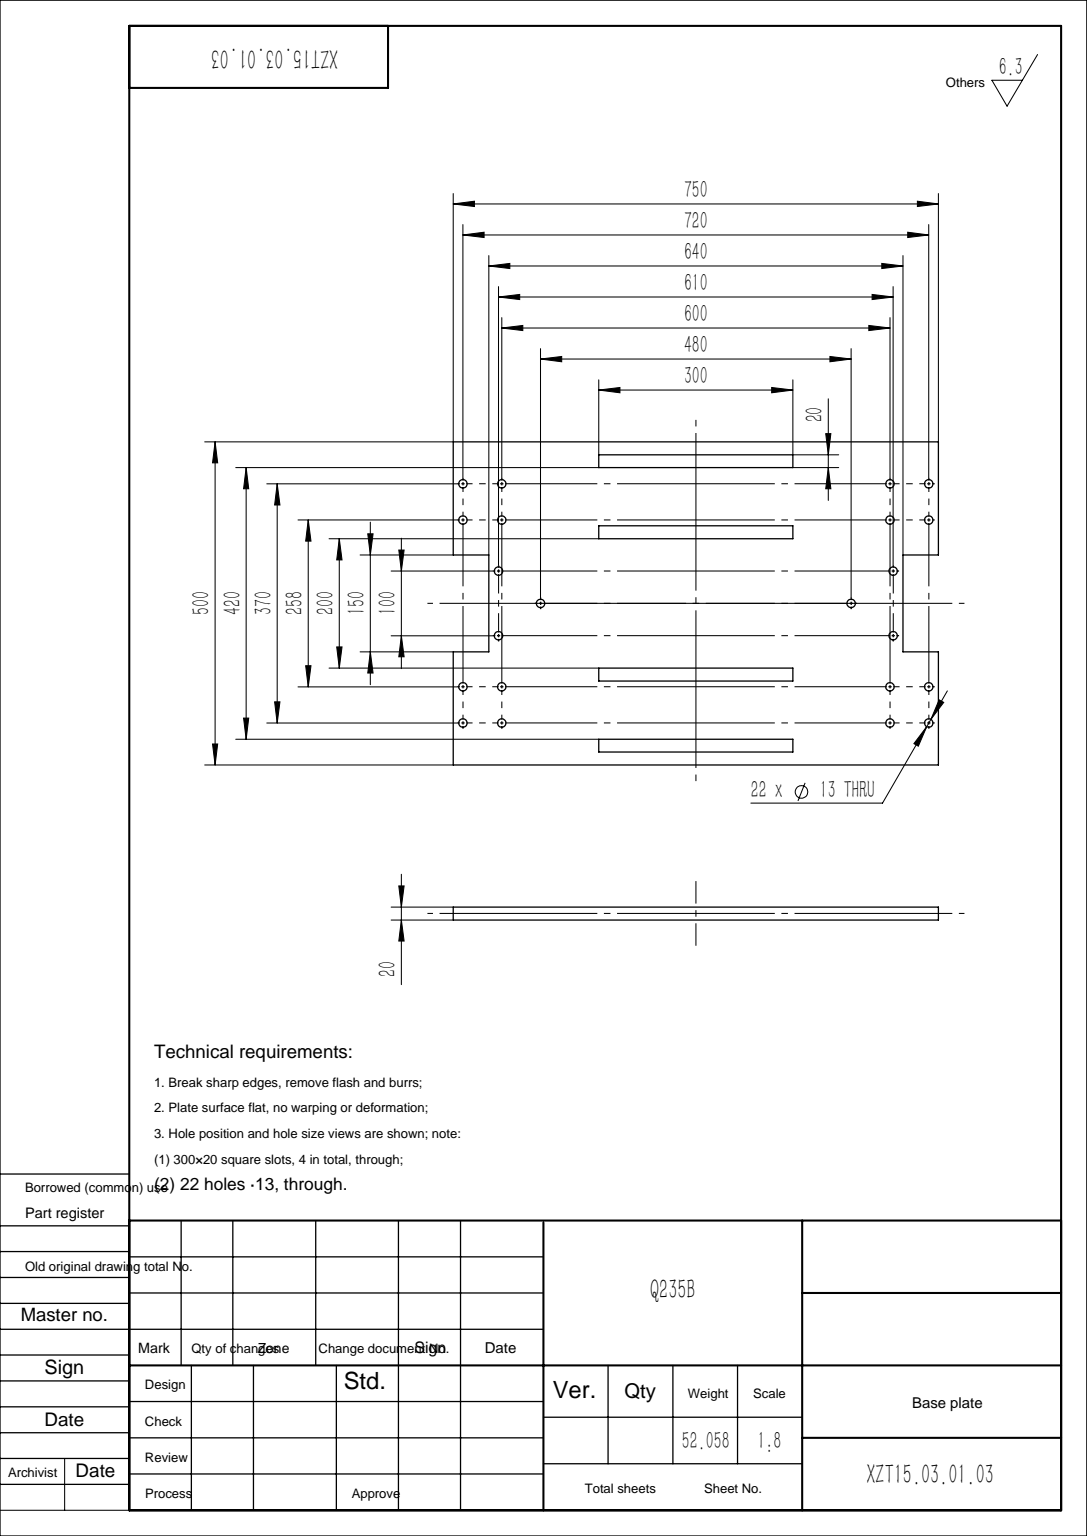
SolidWorks part; units mm, degrees
material "Q235B"
ref_plane "Front Plane" through (0, 0, 0) normal (0, 0, 1) x (1, 0, 0)
ref_plane "Top Plane" through (0, 0, 0) normal (0, 1, 0) x (1, 0, 0)
ref_plane "Right Plane" through (0, 0, 0) normal (1, 0, 0) x (0, 0, -1)
sketch "Sketch1" plane through (0, 0, 0) normal (0, 1, 0) x (1, 0, 0)
  line L0 (0, 0) -> (0, 250) construction
  line L1 (375, -250) -> (-375, -250)
  line L2 (375, -250) -> (375, 250)
  line L3 (375, 250) -> (-375, 250)
  line L4 (-375, -250) -> (-375, 250)
  line L5 (375, -250) -> (-375, 250) construction
  line L6 (375, 250) -> (-375, -250) construction
  line L7 (-320, -75) -> (-430, -75)
  line L8 (-320, -75) -> (-320, 75)
  line L9 (-320, 75) -> (-430, 75)
  line L10 (-430, -75) -> (-430, 75)
  line L11 (-320, -75) -> (-430, 75) construction
  line L12 (-320, 75) -> (-430, -75) construction
  line L13 (0, 0) -> (375, 0) construction
  line L14 (150, -120) -> (-150, -100) construction
  line L15 (150, 210) -> (-150, 210)
  line L16 (150, 210) -> (150, 230)
  line L17 (150, 230) -> (-150, 230)
  line L18 (-150, 210) -> (-150, 230)
  line L19 (150, 210) -> (-150, 230) construction
  line L20 (150, 230) -> (-150, 210) construction
  line L21 (150, 100) -> (-150, 100)
  line L22 (150, 100) -> (150, 120)
  line L23 (150, 120) -> (-150, 120)
  line L24 (-150, 100) -> (-150, 120)
  line L25 (150, 100) -> (-150, 120) construction
  line L26 (150, 120) -> (-150, 100) construction
  line L27 (150, -100) -> (-150, -120) construction
  line L28 (150, -230) -> (-150, -210) construction
  line L29 (150, -210) -> (-150, -230) construction
  line L30 (-150, -100) -> (-150, -120)
  line L31 (150, -120) -> (-150, -120)
  line L32 (150, -100) -> (150, -120)
  line L33 (150, -100) -> (-150, -100)
  line L34 (-150, -210) -> (-150, -230)
  line L35 (150, -230) -> (-150, -230)
  line L36 (150, -210) -> (150, -230)
  line L37 (150, -210) -> (-150, -210)
  line L38 (320, 75) -> (430, -75) construction
  line L39 (320, -75) -> (430, 75) construction
  line L40 (430, -75) -> (430, 75)
  line L41 (320, 75) -> (430, 75)
  line L42 (320, -75) -> (320, 75)
  line L43 (320, -75) -> (430, -75)
  point P0 (0, 0)
  point P5 (-375, 0)
  point P14 (0, 220)
  point P19 (0, 110)
  point P32 (0, -110)
  point P33 (0, -220)
  dimension "D1" = 500
  dimension "D2" = 750
  dimension "D3" = 150
  dimension "D4" = 110
  dimension "D5" = 20
  dimension "D6" = 300
  dimension "D7" = 200
  dimension "D8" = 420
extrude "Boss-Extrude1" add sketch "Sketch1" along normal blind 20 contours L43 L42 L41 L2 L3 L4 L9 L8 L7 L1 L37 L36 L35 L34 L33 L32 L31 L30 L15 L18 L17 L16 L21 L24 L23 L22
hole_wizard "Ø13.0 (13) Diameter Hole1" positions "Sketch2" profile "Sketch3" hole size "Ø13.0" standard "GB" end condition up to next
sketch "Sketch2" plane through (0, 20, 0) normal (0, 1, 0) x (1, 0, 0)
  line L0 (-240, 0) -> (0, 0) construction
  line L1 (0, 0) -> (0, 250) construction
  line L2 (375, 250) -> (-375, 250) construction
  line L4 (-360, 129) -> (-300, 129) construction
  line L5 (-360, 129) -> (-360, 185) construction
  line L6 (-360, -129) -> (-360, -185) construction
  line L7 (-360, -129) -> (-300, -129) construction
  line L8 (360, -129) -> (300, -129) construction
  line L9 (360, -129) -> (360, -185) construction
  line L10 (360, 129) -> (360, 185) construction
  line L11 (360, 129) -> (300, 129) construction
  point P0 (-360, 129)
  point P2 (-305, 50)
  point P4 (-240, 0)
  point P19 (-300, 129)
  point P20 (-300, 185)
  point P21 (-360, 185)
  point P26 (-360, -129)
  point P27 (-360, -185)
  point P28 (-300, -129)
  point P29 (-300, -185)
  point P30 (-305, -50)
  point P38 (360, -129)
  point P39 (300, -129)
  point P40 (360, -185)
  point P41 (360, 129)
  point P42 (360, 185)
  point P43 (300, 129)
  point P44 (305, -50)
  point P45 (300, -185)
  point P46 (300, 185)
  point P47 (240, 0)
  point P48 (305, 50)
  dimension "D1" = 480
  dimension "D2" = 610
  dimension "D5" = 90
  dimension "D6" = 60
  dimension "D7" = 56
  dimension "D8" = 600
  dimension "D9" = 258
  dimension "D10" = 100
  dimension "D3" = 2
  dimension "D4" = 2
sketch "Sketch3" plane through (-360, 20, -129) normal (1, 0, 0) x (0, 0, 1)
  line L0 (0, 0) -> (0, 20)
  line L1 (0, 20) -> (6.5, 20)
  line L2 (6.5, 20) -> (6.5, 0)
  line L5 (6.5, 0) -> (0, 0)
  line L11 (0, -6.35) -> (0, 107.95) construction
  dimension "通孔孔直径" = 13
  dimension "通孔孔深度" = 20
